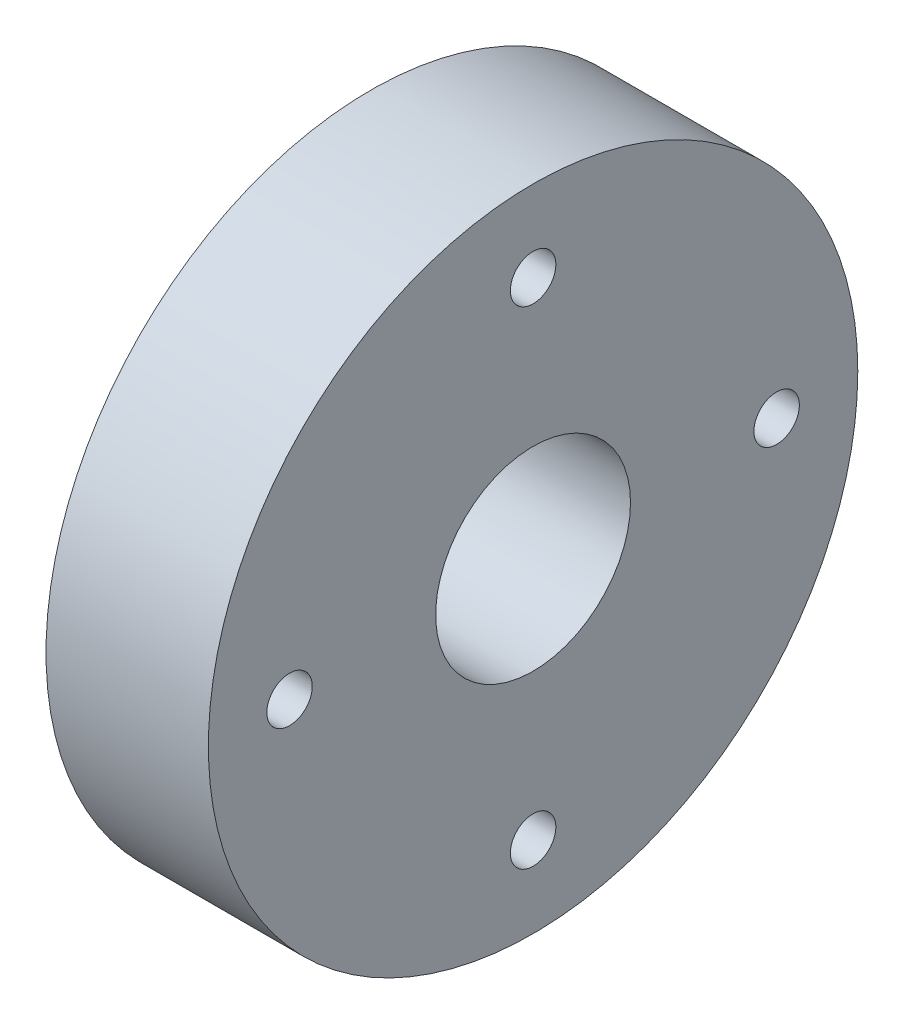
from build123d import *

# Parameters (mm, degrees)
SKETCH1_W          = 50
SKETCH1_H          = 70
M16_TAPPED_HOLE1_D = 14
CIRPATTERN1_COUNT  = 4


with BuildPart() as part:
    # Sketch1 → Revolve1 (revolve)
    with BuildSketch(Plane.XY, mode=Mode.PRIVATE) as revolve1_sk:
        with Locations((0, 65)):
            Rectangle(SKETCH1_W, SKETCH1_H)
    revolve(revolve1_sk.sketch.rotate(Axis((71.901236476, 0, 0), (-1, 0, 0)), 90), axis=Axis((71.901236476, 0, 0), (-1, 0, 0)))

    # M16 Tapped Hole1 (through all)
    with Locations(Plane(origin=(-25, 0, -75), x_dir=(0, 0, -1), z_dir=(-1, 0, 0))):
        with Locations((0, 0)):
            m16_tapped_hole1 = Hole(M16_TAPPED_HOLE1_D / 2)

    # CirPattern1: M16 Tapped Hole1 ×4 about axis
    cirpattern1_axis = Axis((0, 0, 0), (1, 0, 0))
    for i in range(1, CIRPATTERN1_COUNT):
        add(m16_tapped_hole1.rotate(cirpattern1_axis, i * 360 / CIRPATTERN1_COUNT), mode=Mode.SUBTRACT)


solid = part.part
